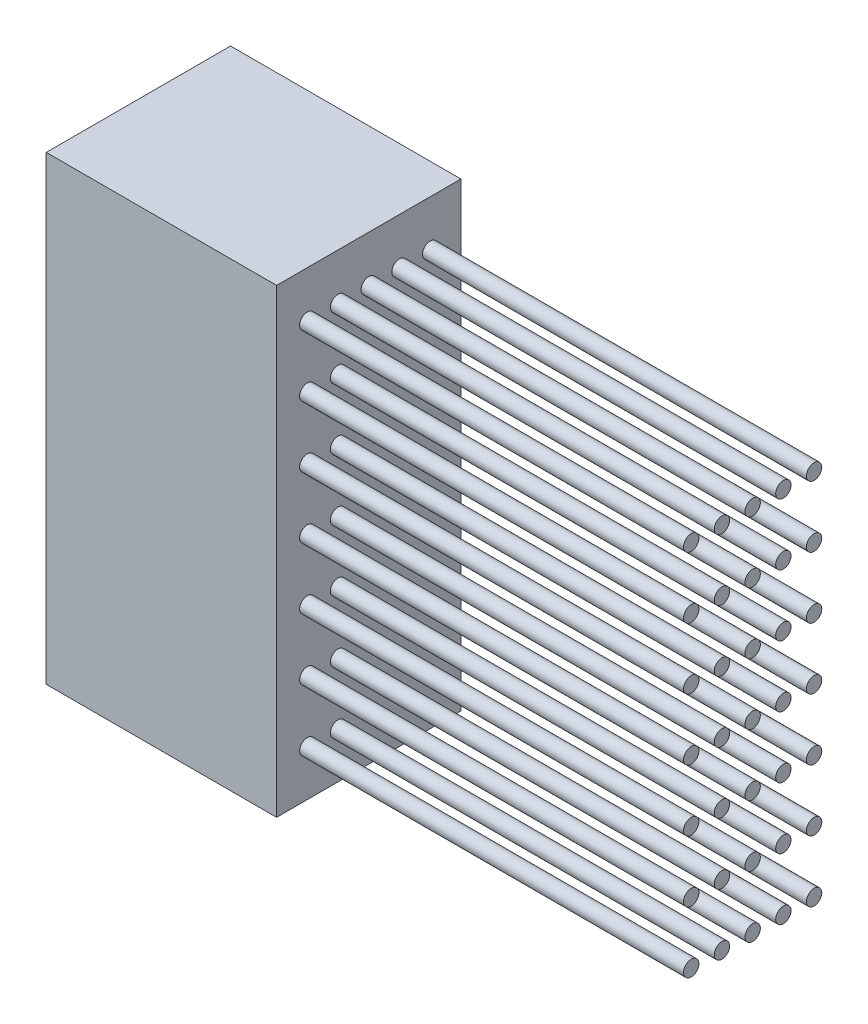
from build123d import *

# Parameters (mm, degrees)
SKETCH_1_W               = 15
SKETCH_1_H               = 30
EXTRUDE_1_DEPTH          = 6
SKETCH_2_R               = 0.5
EXTRUDE_2_DEPTH          = 25
PATTERN_LINEAR_1_COUNT   = 4
PATTERN_LINEAR_1_PITCH   = 4
MIRROR_1_COPY_1_SKETCH_R = 0.5
MIRROR_1_COPY_1_DEPTH    = 25
MIRROR_1_COPY_2_SKETCH_R = 0.5
MIRROR_1_COPY_2_DEPTH    = 25
MIRROR_1_COPY_3_SKETCH_R = 0.5
MIRROR_1_COPY_3_DEPTH    = 25
MIRROR_1_COPY_4_SKETCH_R = 0.5
MIRROR_1_COPY_4_DEPTH    = 25


with BuildPart() as part:
    # 草图1 → 凸台-拉伸1 (new, symmetric)
    with BuildSketch(Plane.XY):
        Rectangle(SKETCH_1_W, SKETCH_1_H)
    extrude(amount=EXTRUDE_1_DEPTH, both=True)

    # 草图2 → 凸台-拉伸2 (add)
    with BuildSketch(Plane(origin=(7.5, 0, 0), x_dir=(0, 0, -1), z_dir=(1, 0, 0))):
        with Locations(Location((-4, 0, 0), (0, 0, 180))):
            Circle(SKETCH_2_R)
        with Locations(Location((-2, 0, 0), (0, 0, 180))):
            Circle(SKETCH_2_R)
        with Locations(Location((0, 0, 0), (0, 0, 180))):
            Circle(SKETCH_2_R)
        with Locations(Location((2, 0, 0), (0, 0, 180))):
            Circle(SKETCH_2_R)
        with Locations(Location((4, 0, 0), (0, 0, 180))):
            Circle(SKETCH_2_R)
    extrude_2 = extrude(amount=EXTRUDE_2_DEPTH)

    # 阵列(线性)1: 凸台-拉伸2 ×4
    with Locations(*[(0, -i * PATTERN_LINEAR_1_PITCH, 0) for i in range(1, PATTERN_LINEAR_1_COUNT)]):
        add(extrude_2)

    # 镜向1 copy 1 sketch → 镜向1 copy 1 (add)
    with BuildSketch(Plane(origin=(7.5, 4, 0), x_dir=(0, 0, -1), z_dir=(1, 0, 0))):
        with Locations((-4, 0)):
            Circle(MIRROR_1_COPY_1_SKETCH_R)
        with Locations((-2, 0)):
            Circle(MIRROR_1_COPY_1_SKETCH_R)
        Circle(MIRROR_1_COPY_1_SKETCH_R)
        with Locations((2, 0)):
            Circle(MIRROR_1_COPY_1_SKETCH_R)
        with Locations((4, 0)):
            Circle(MIRROR_1_COPY_1_SKETCH_R)
    extrude(amount=MIRROR_1_COPY_1_DEPTH)

    # 镜向1 copy 2 sketch → 镜向1 copy 2 (add)
    with BuildSketch(Plane(origin=(7.5, 8, 0), x_dir=(0, 0, -1), z_dir=(1, 0, 0))):
        with Locations((-4, 0)):
            Circle(MIRROR_1_COPY_2_SKETCH_R)
        with Locations((-2, 0)):
            Circle(MIRROR_1_COPY_2_SKETCH_R)
        Circle(MIRROR_1_COPY_2_SKETCH_R)
        with Locations((2, 0)):
            Circle(MIRROR_1_COPY_2_SKETCH_R)
        with Locations((4, 0)):
            Circle(MIRROR_1_COPY_2_SKETCH_R)
    extrude(amount=MIRROR_1_COPY_2_DEPTH)

    # 镜向1 copy 3 sketch → 镜向1 copy 3 (add)
    with BuildSketch(Plane(origin=(7.5, 12, 0), x_dir=(0, 0, -1), z_dir=(1, 0, 0))):
        with Locations((-4, 0)):
            Circle(MIRROR_1_COPY_3_SKETCH_R)
        with Locations((-2, 0)):
            Circle(MIRROR_1_COPY_3_SKETCH_R)
        Circle(MIRROR_1_COPY_3_SKETCH_R)
        with Locations((2, 0)):
            Circle(MIRROR_1_COPY_3_SKETCH_R)
        with Locations((4, 0)):
            Circle(MIRROR_1_COPY_3_SKETCH_R)
    extrude(amount=MIRROR_1_COPY_3_DEPTH)

    # 镜向1 copy 4 sketch → 镜向1 copy 4 (add)
    with BuildSketch(Plane(origin=(7.5, 0, 0), x_dir=(0, 0, -1), z_dir=(1, 0, 0))):
        with Locations((-4, 0)):
            Circle(MIRROR_1_COPY_4_SKETCH_R)
        with Locations((-2, 0)):
            Circle(MIRROR_1_COPY_4_SKETCH_R)
        Circle(MIRROR_1_COPY_4_SKETCH_R)
        with Locations((2, 0)):
            Circle(MIRROR_1_COPY_4_SKETCH_R)
        with Locations((4, 0)):
            Circle(MIRROR_1_COPY_4_SKETCH_R)
    extrude(amount=MIRROR_1_COPY_4_DEPTH)


solid = part.part
